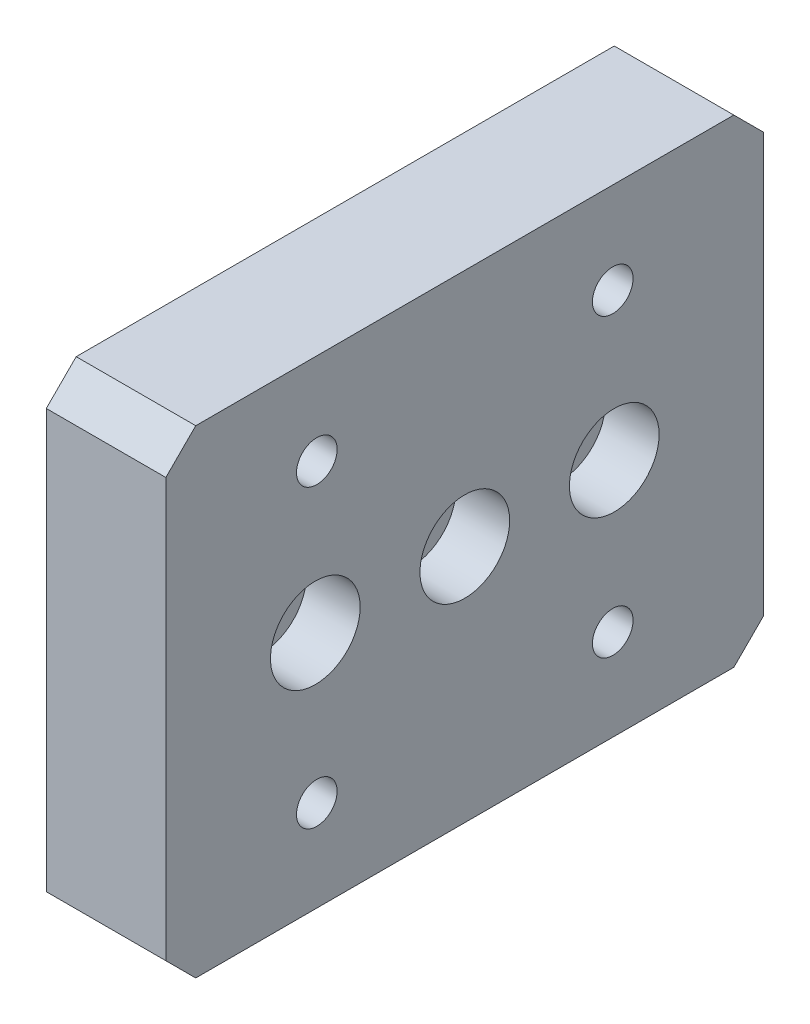
from build123d import *

# Parameters (mm, degrees)
SKETCH_1_W                = 100
SKETCH_1_H                = 80
EXTRUDE_1_DEPTH           = 20
HOLE_WIZARD_M8_1_D        = 6.8
HOLE_WIZARD_1_D           = 9
HOLE_WIZARD_1_CBORE_D     = 15
HOLE_WIZARD_1_CBORE_DEPTH = 9
CHAMFER_1_SIZE            = 5


with BuildPart() as part:
    # 草图1 → 凸台-拉伸1 (new body)
    with BuildSketch(Plane(origin=(0, 0, 0), x_dir=(0, 0, -1), z_dir=(1, 0, 0))):
        Rectangle(SKETCH_1_W, SKETCH_1_H)
    extrude(amount=EXTRUDE_1_DEPTH)

    # M8 螺纹孔1 (through all)
    with Locations(Plane(origin=(20, 0, 0), x_dir=(0, 0, -1), z_dir=(1, 0, 0))):
        with Locations((-24.748737342, 24.748737342), (24.748737342, 24.748737342), (24.748737342, -24.748737342), (-24.748737342, -24.748737342)):
            Hole(HOLE_WIZARD_M8_1_D / 2)

    # 打孔尺寸(%根据)内六角圆柱头螺钉的类型1 (through all)
    with Locations(Plane(origin=(20, 0, 0), x_dir=(0, 0, -1), z_dir=(1, 0, 0))):
        with Locations((-25, 0), (0, 0), (25, 0)):
            CounterBoreHole(HOLE_WIZARD_1_D / 2, HOLE_WIZARD_1_CBORE_D / 2, HOLE_WIZARD_1_CBORE_DEPTH)

    # 倒角1
    chamfer_1_edges = [part.edges().sort_by_distance(p)[0] for p in [
        (10, -40, -50),
        (10, -40, 50),
        (10, 40, 50),
        (10, 40, -50),
    ]]
    chamfer(chamfer_1_edges, length=CHAMFER_1_SIZE)


solid = part.part
